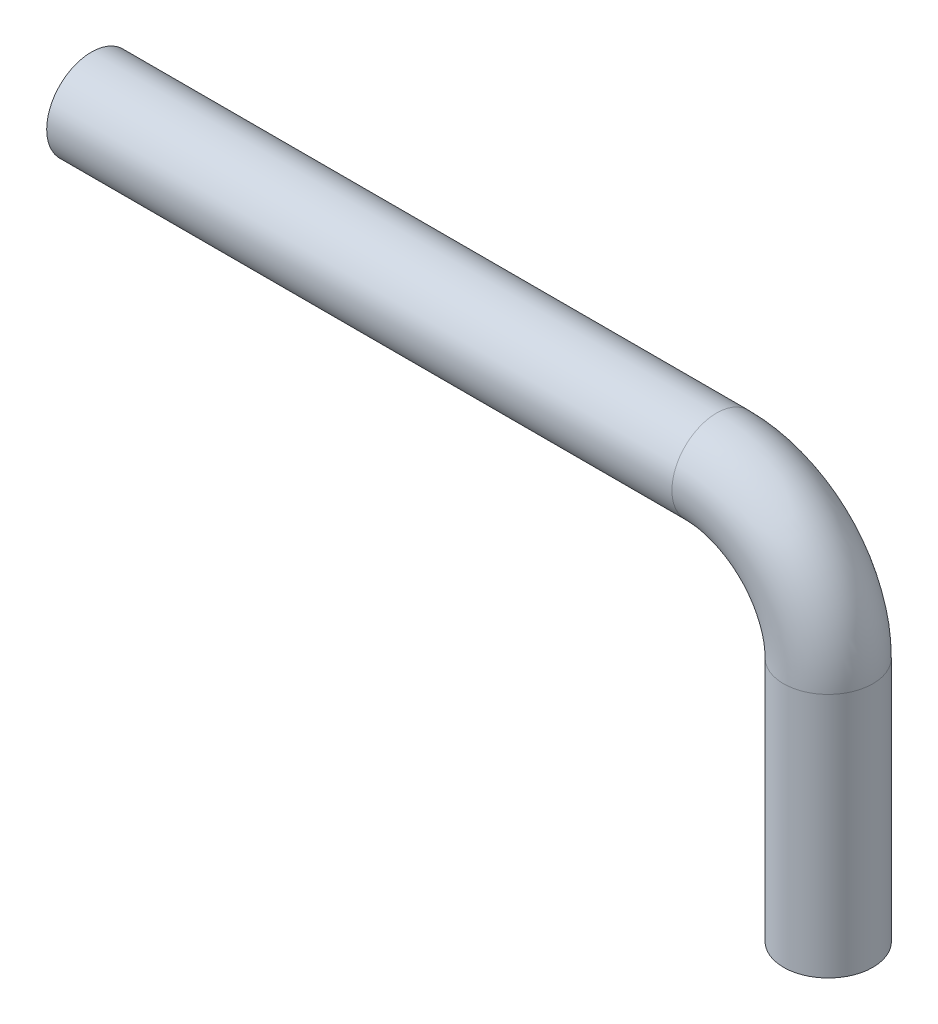
SolidWorks part; units mm, degrees
ref_plane "Front Plane" through (0, 0, 0) normal (0, 0, 1) x (1, 0, 0)
ref_plane "Top Plane" through (0, 0, 0) normal (0, 1, 0) x (1, 0, 0)
ref_plane "Right Plane" through (0, 0, 0) normal (1, 0, 0) x (0, 0, -1)
sketch "Sketch1" plane through (0, 0, 0) normal (0, 0, 1) x (1, 0, 0)
  line L0 (0, 0) -> (28, 0)
  line L1 (33, -5) -> (33, -16)
  arc A0 (28, 0) -> (33, -5) centre (28, -5) cw
  point P6 (33, 0)
  dimension "D3" = 5
  dimension "D1" = 33
  dimension "D2" = 16
sweep "Sweep1" add path "Sketch1" circular profile diameter 4 parameters "D3"=4
cosmetic thread "Cosmetic Thread1" parameters "D1"=20, "D2"=3.999
